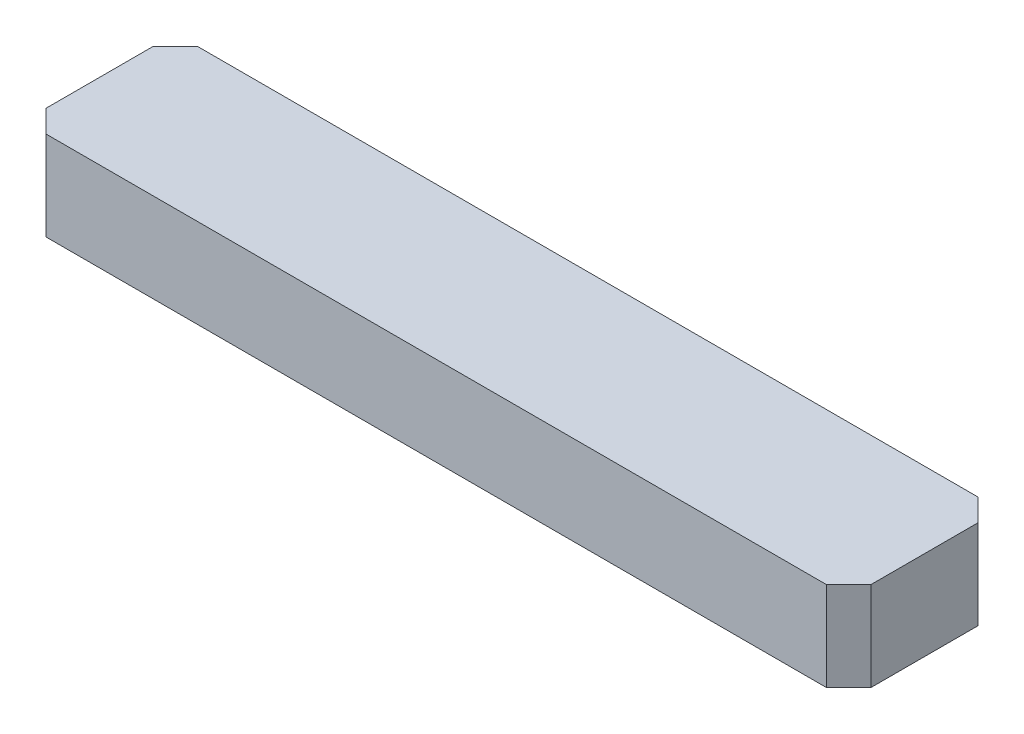
from build123d import *

# Parameters (mm, degrees)
SKETCH1_W           = 37
SKETCH1_H           = 6.8
BOSS_EXTRUDE1_DEPTH = 2
CHAMFER1_SIZE       = 1


with BuildPart() as part:
    # Sketch1 → Boss-Extrude1 (new, symmetric)
    with BuildSketch(Plane(origin=(0, 0, 0), x_dir=(1, 0, 0), z_dir=(0, 1, 0))):
        Rectangle(SKETCH1_W, SKETCH1_H)
    extrude(amount=BOSS_EXTRUDE1_DEPTH, both=True)

    # Chamfer1
    chamfer1_edges = [part.edges().sort_by_distance(p)[0] for p in [
        (18.5, 0, 3.4),
        (-18.5, 0, 3.4),
        (-18.5, 0, -3.4),
        (18.5, 0, -3.4),
    ]]
    chamfer(chamfer1_edges, length=CHAMFER1_SIZE)


solid = part.part
